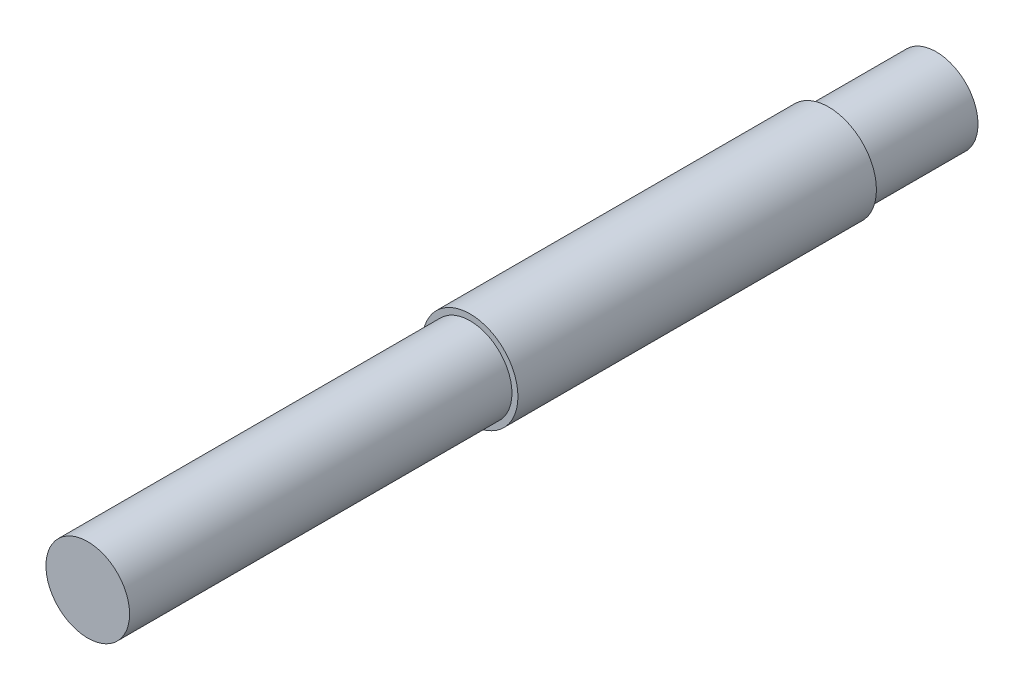
SolidWorks part; units mm, degrees
ref_plane "前视基准面" through (0, 0, 0) normal (0, 0, 1) x (1, 0, 0)
ref_plane "上视基准面" through (0, 0, 0) normal (0, 1, 0) x (1, 0, 0)
ref_plane "右视基准面" through (0, 0, 0) normal (1, 0, 0) x (0, 0, -1)
sketch "草图1" plane through (0, 0, 0) normal (0, 0, 1) x (1, 0, 0)
  circle A0 centre (0, 0) radius 20
  dimension "D1" = 40
extrude "凸台-拉伸1" add sketch "草图1" along normal blind 150
sketch "草图2" plane through (0, 0, 150) normal (0, 0, 1) x (1, 0, 0)
  circle A0 centre (0, 0) radius 17.5
  dimension "D1" = 35
extrude "凸台-拉伸2" add sketch "草图2" along normal blind 160
sketch "草图3" plane through (0, 0, 0) normal (0, 0, -1) x (-1, 0, 0)
  circle A0 centre (0, 0) radius 17.5
  dimension "D1" = 35
extrude "凸台-拉伸3" add sketch "草图3" along normal blind 45
